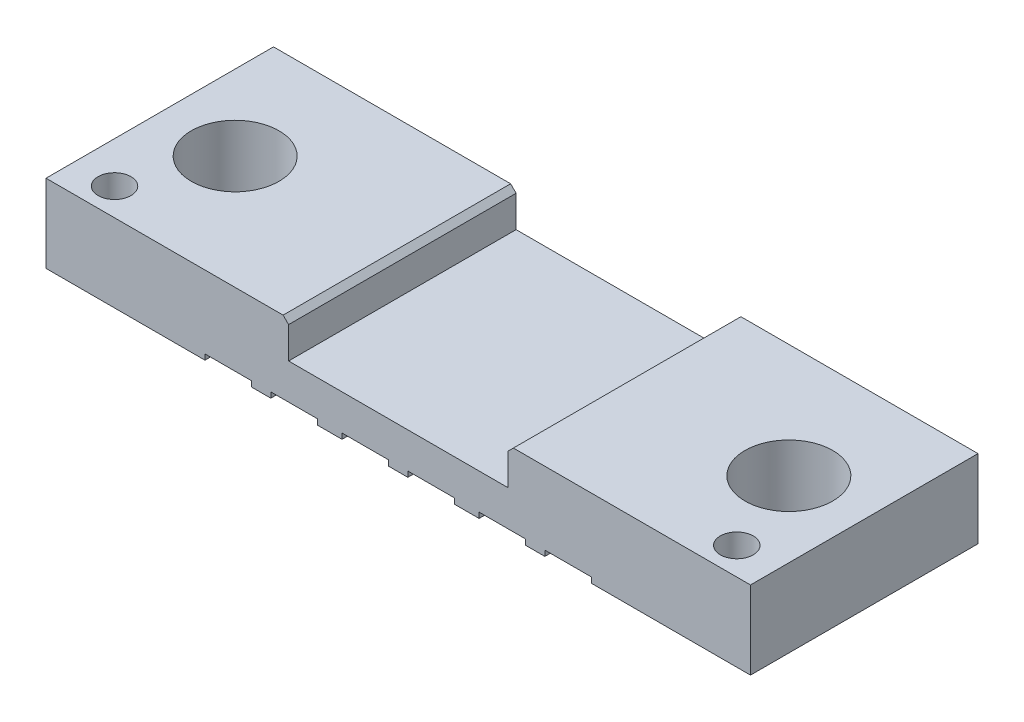
from build123d import *

# Parameters (mm, degrees)
SKETCH1_W           = 25.7
SKETCH1_H           = 8.3
BOSS_EXTRUDE1_DEPTH = 2.85
SKETCH2_R           = 1.6
SKETCH2_R_2         = 0.6
CUT_EXTRUDE1_DEPTH  = 14.800996341
SKETCH3_W           = 1.7
SKETCH3_H           = 8.3
CUT_EXTRUDE2_DEPTH  = 0.2
SKETCH4_W           = 8
SKETCH4_H           = 8.3
CUT_EXTRUDE3_DEPTH  = 1.35
CHAMFER1_SIZE       = 0.2


with BuildPart() as part:
    # Sketch1 → Boss-Extrude1 (new body)
    with BuildSketch(Plane(origin=(0, 0, 0), x_dir=(1, 0, 0), z_dir=(0, 1, 0))):
        Rectangle(SKETCH1_W, SKETCH1_H)
    extrude(amount=BOSS_EXTRUDE1_DEPTH)

    # Sketch2 → Cut-Extrude1 (cut, through all)
    with BuildSketch(Plane(origin=(0, 2.85, 0), x_dir=(1, 0, 0), z_dir=(0, 1, 0))):
        with Locations(Location((-10.1, 0, 0), (0, 0, 270))):
            Circle(SKETCH2_R)
        with Locations(Location((-11.35, -3.15, 0), (0, 0, 270))):
            Circle(SKETCH2_R_2)
        with Locations(Location((10.1, 0, 0), (0, 0, 90))):
            Circle(SKETCH2_R)
        with Locations(Location((11.35, -3.15, 0), (0, 0, 90))):
            Circle(SKETCH2_R_2)
    extrude(amount=-CUT_EXTRUDE1_DEPTH, mode=Mode.SUBTRACT)

    # Sketch3 → Cut-Extrude2 (cut)
    with BuildSketch(Plane.XZ):
        with Locations((-6.2, 0)):
            Rectangle(SKETCH3_W, SKETCH3_H)
        with Locations((1.2, 0)):
            Rectangle(SKETCH3_W, SKETCH3_H)
        with Locations((-3.8, 0)):
            Rectangle(SKETCH3_W, SKETCH3_H)
        with Locations((-1.2, 0)):
            Rectangle(SKETCH3_W, SKETCH3_H)
        with Locations((3.8, 0)):
            Rectangle(SKETCH3_W, SKETCH3_H)
        with Locations((6.2, 0)):
            Rectangle(SKETCH3_W, SKETCH3_H)
    extrude(amount=-CUT_EXTRUDE2_DEPTH, mode=Mode.SUBTRACT)

    # Sketch4 → Cut-Extrude3 (cut)
    with BuildSketch(Plane(origin=(0, 2.85, 0), x_dir=(1, 0, 0), z_dir=(0, 1, 0))):
        Rectangle(SKETCH4_W, SKETCH4_H)
    extrude(amount=-CUT_EXTRUDE3_DEPTH, mode=Mode.SUBTRACT)

    # Chamfer1
    chamfer1_edges = [part.edges().sort_by_distance(p)[0] for p in [
        (4, 2.85, 0),
        (-4, 2.85, 0),
    ]]
    chamfer(chamfer1_edges, length=CHAMFER1_SIZE)


solid = part.part
